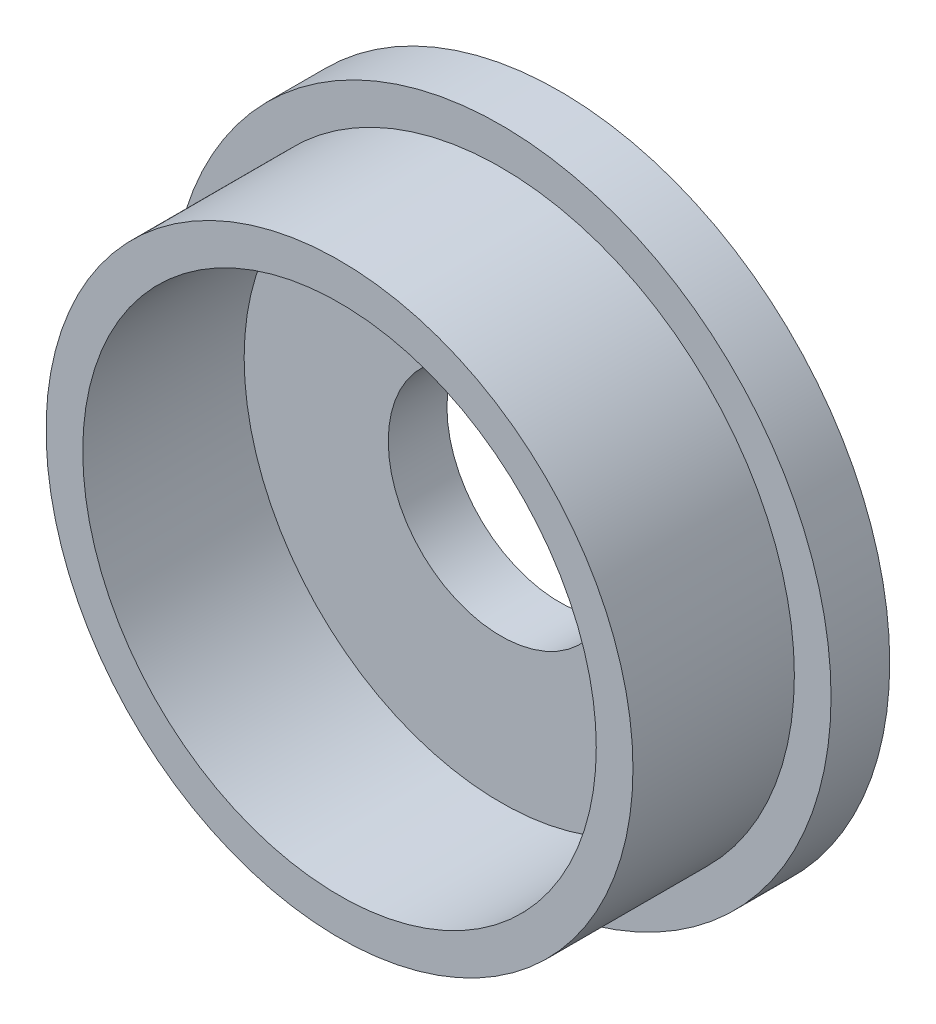
SolidWorks part; units mm, degrees
ref_plane "前视基准面" through (0, 0, 0) normal (0, 0, 1) x (1, 0, 0)
ref_plane "上视基准面" through (0, 0, 0) normal (0, 1, 0) x (1, 0, 0)
ref_plane "右视基准面" through (0, 0, 0) normal (1, 0, 0) x (0, 0, -1)
sketch "草图1" plane through (0, 0, 0) normal (0, 0, 1) x (1, 0, 0)
  circle A0 centre (0, 0) radius 22.5
  dimension "D2" = 45
extrude "凸台-拉伸1" add sketch "草图1" along normal mid plane 4
sketch "草图2" plane through (0, 0, 2) normal (0, 0, 1) x (1, 0, 0)
  circle A0 centre (0, 0) radius 17.5
  circle A1 centre (0, 0) radius 20
  dimension "D1" = 35
  dimension "D2" = 40
extrude "凸台-拉伸2" add sketch "草图2" along normal blind 11
sketch "草图3" plane through (0, 0, 2) normal (0, 0, 1) x (1, 0, 0)
  circle A0 centre (0, 0) radius 7.6787
extrude "切除-拉伸1" cut sketch "草图3" against normal blind 21
